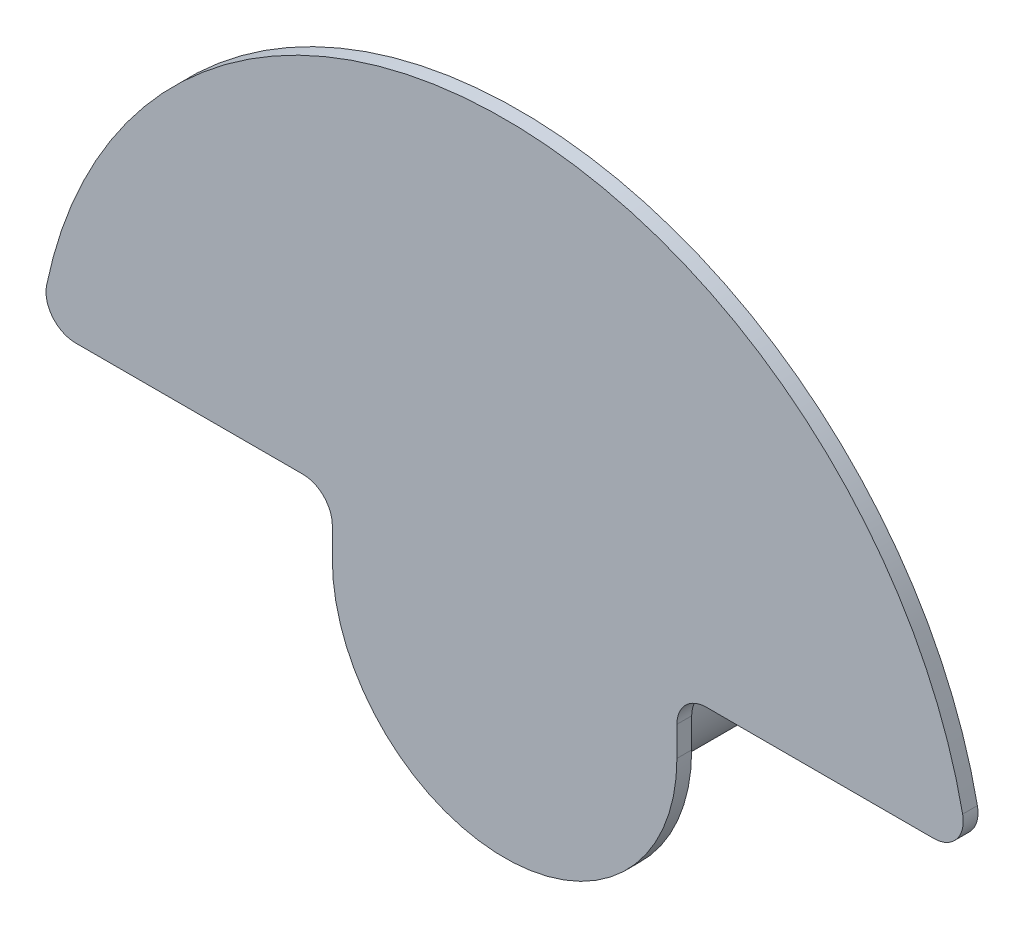
from build123d import *

# Parameters (mm, degrees)
EXTRUDE_1_DEPTH             = 1.5
SKETCH_2_W                  = 12.5
SKETCH_2_H                  = 13.5
HOLE_WIZARD_12_0_12_1_D     = 12
HOLE_WIZARD_12_0_12_1_DEPTH = 13.5
SKETCH_5_W                  = 1.65
SKETCH_5_H                  = 11.731334643
HOLE_WIZARD_3_3_3_3_2_D     = 3.3
HOLE_WIZARD_3_3_3_3_2_DEPTH = 41.731334643
FILLET_1_R                  = 3


with BuildPart() as part:
    # 草图1 → 凸台-拉伸1 (new body)
    with BuildSketch(Plane.XY.offset(0.75)):
        with BuildLine():
            Line((17.5, 6), (47.11952886, 6))
            ThreePointArc((47.11952886, 6), (0, 47.5), (-47.11952886, 6))
            Line((-47.11952886, 6), (-17.5, 6))
            Line((-17.5, 6), (-17.5, 0))
            ThreePointArc((-17.5, 0), (0, -17.5), (17.5, 0))
            Line((17.5, 0), (17.5, 6))
        make_face()
    extrude(amount=-EXTRUDE_1_DEPTH)

    # 草图2 → 旋转1 (revolve)
    with BuildSketch(Plane(origin=(0, 0, 0), x_dir=(1, 0, 0), z_dir=(0, 1, 0))):
        with Locations((6.25, 7.5)):
            Rectangle(SKETCH_2_W, SKETCH_2_H)
    revolve(axis=Axis((0, 0, -14.25), (0, 0, 1)))

    # Ø12.0 (12) 直径孔1
    with Locations(Plane(origin=(0, 0, -14.25), x_dir=(-1, 0, 0), z_dir=(0, 0, -1))):
        with Locations((0, 0)):
            Hole(HOLE_WIZARD_12_0_12_1_D / 2, depth=HOLE_WIZARD_12_0_12_1_DEPTH)

    # 草图5 → Ø3.3 (3.3) 直径孔1 (revolve, cut)
    with BuildSketch(Plane(origin=(0, -5.768665357, -9.25), x_dir=(0, 0, 1), z_dir=(1, 0, 0))):
        with Locations((0.825, 5.865667322)):
            Rectangle(SKETCH_5_W, SKETCH_5_H)
    revolve(axis=Axis((0, 0.581334643, -9.25), (0, -1, 0)), mode=Mode.SUBTRACT)

    # Ø3.3 (3.3) 直径孔2
    with Locations(Plane(origin=(0, 5.768665357, 0), x_dir=(-1, 0, 0), z_dir=(0, -1, 0))):
        with Locations((0, 9.25)):
            Hole(HOLE_WIZARD_3_3_3_3_2_D / 2, depth=HOLE_WIZARD_3_3_3_3_2_DEPTH)

    # 圆角1
    fillet_1_edges = [part.edges().sort_by_distance(p)[0] for p in [
        (-17.5, 6, 0),
        (-47.11952886, 6, 0),
        (47.11952886, 6, 0),
        (17.5, 6, 0),
    ]]
    fillet(fillet_1_edges, radius=FILLET_1_R)


solid = part.part
